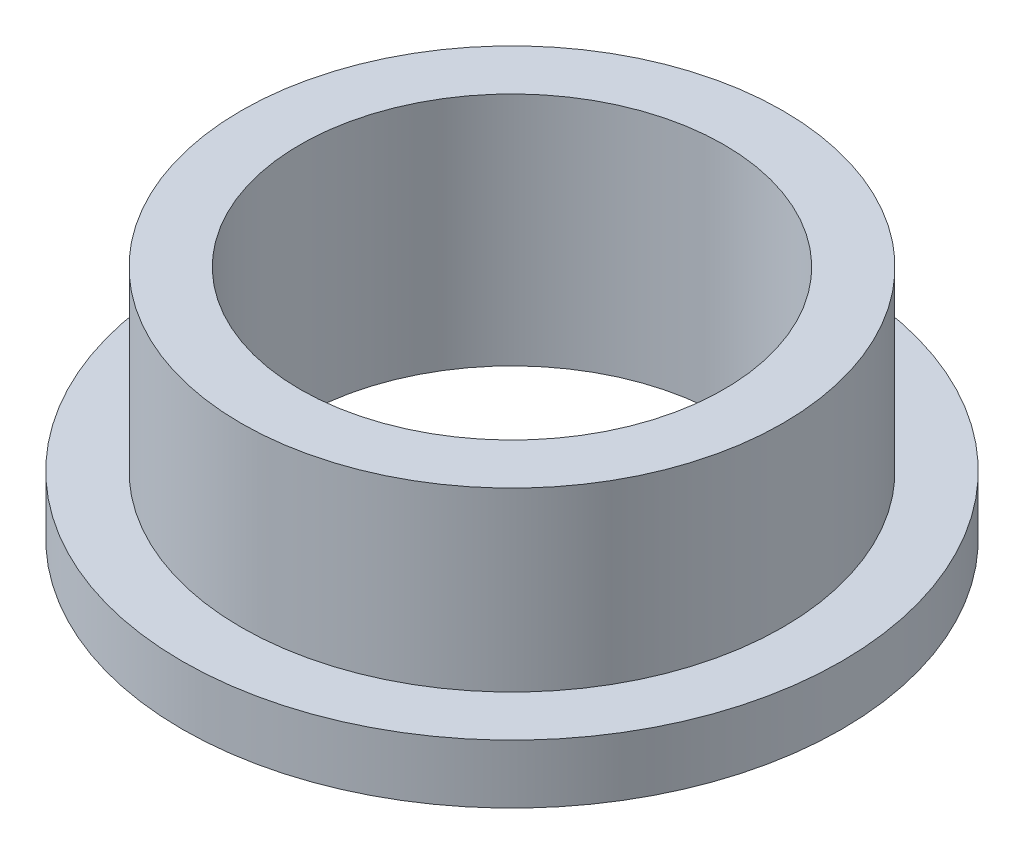
SolidWorks part; units mm, degrees
ref_plane "前视基准面" through (0, 0, 0) normal (0, 0, 1) x (1, 0, 0)
ref_plane "上视基准面" through (0, 0, 0) normal (0, 1, 0) x (1, 0, 0)
ref_plane "右视基准面" through (0, 0, 0) normal (1, 0, 0) x (0, 0, -1)
sketch "草图1" plane through (0, 0, 0) normal (0, 1, 0) x (1, 0, 0)
  circle A0 centre (0, 0) radius 28
  circle A1 centre (0, 0) radius 18
extrude "凸台-拉伸1" add sketch "草图1" along normal blind 5
sketch "草图2" plane through (0, 5, 0) normal (0, 1, 0) x (1, 0, 0)
  circle A0 centre (0, 0) radius 18
  circle A1 centre (0, 0) radius 23
extrude "凸台-拉伸2" add sketch "草图2" along normal blind 15
